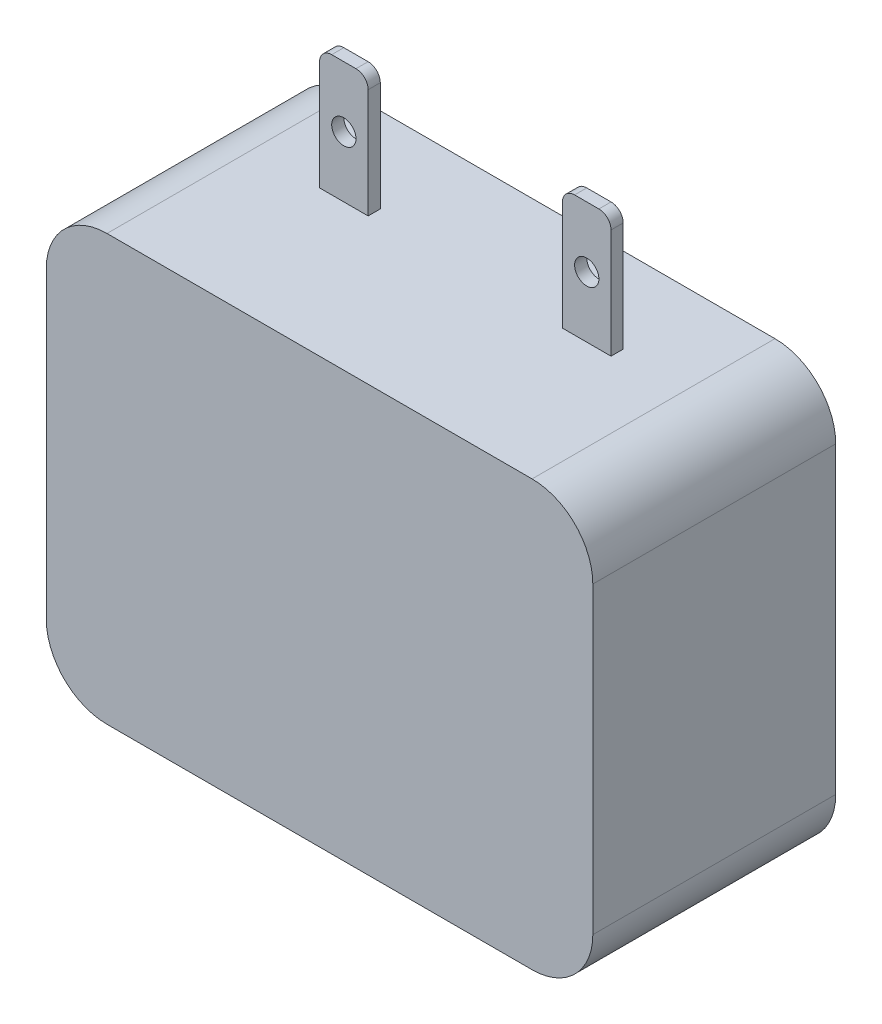
SolidWorks part; units mm, degrees
ref_plane "Front Plane" through (0, 0, 0) normal (0, 0, 1) x (1, 0, 0)
ref_plane "Top Plane" through (0, 0, 0) normal (0, 1, 0) x (1, 0, 0)
ref_plane "Right Plane" through (0, 0, 0) normal (1, 0, 0) x (0, 0, -1)
sketch "Sketch1" plane through (0, 0, 0) normal (0, 0, 1) x (1, 0, 0)
  line L1 (-17.5, -17.5) -> (17.5, -17.5)
  line L2 (-22.5, -12.5) -> (-22.5, 12.5)
  line L3 (-17.5, 17.5) -> (17.5, 17.5)
  line L4 (22.5, -12.5) -> (22.5, 12.5)
  line L5 (-22.5, -17.5) -> (22.5, 17.5) construction
  line L6 (-22.5, 17.5) -> (22.5, -17.5) construction
  arc A0 (-17.5, -17.5) -> (-22.5, -12.5) centre (-17.5, -12.5) cw
  arc A1 (17.5, -17.5) -> (22.5, -12.5) centre (17.5, -12.5) ccw
  arc A2 (17.5, 17.5) -> (22.5, 12.5) centre (17.5, 12.5) cw
  arc A3 (-22.5, 12.5) -> (-17.5, 17.5) centre (-17.5, 12.5) cw
  point P0 (0, 0)
  dimension "D3" = 5
  dimension "D1" = 35
  dimension "D2" = 45
extrude "Boss-Extrude1" add sketch "Sketch1" along normal mid plane 20
ref_plane "Plane1" through (0, 0, -3) normal (0, 0, -1) x (-1, 0, 0)
sketch "Sketch3" plane through (0, 0, -3) normal (0, 0, -1) x (-1, 0, 0)
  line L0 (-17.5, 17.5) -> (17.5, 17.5) construction
  line L4 (-8, 17.5) -> (-12, 17.5)
  line L5 (-8, 17.5) -> (-8, 26.5)
  line L6 (-9, 27.5) -> (-11, 27.5)
  line L7 (-12, 17.5) -> (-12, 26.5)
  line L8 (0, 11) -> (0, -11) construction
  line L9 (8, 17.5) -> (12, 17.5)
  line L10 (9, 27.5) -> (11, 27.5)
  line L11 (8, 17.5) -> (8, 26.5)
  line L12 (12, 17.5) -> (12, 26.5)
  line L13 (17.5, -17.5) -> (-17.5, -17.5) construction
  line L14 (-2.5, -17.5) -> (2.5, -17.5)
  line L15 (-2.5, -17.5) -> (-2.5, -26.5)
  line L16 (-1.5, -27.5) -> (1.5, -27.5)
  line L17 (2.5, -17.5) -> (2.5, -26.5)
  arc A2 (-8, 26.5) -> (-9, 27.5) centre (-9, 26.5) ccw
  arc A3 (-11, 27.5) -> (-12, 26.5) centre (-11, 26.5) ccw
  arc A4 (11, 27.5) -> (12, 26.5) centre (11, 26.5) cw
  arc A5 (8, 26.5) -> (9, 27.5) centre (9, 26.5) cw
  arc A6 (-2.5, -26.5) -> (-1.5, -27.5) centre (-1.5, -26.5) ccw
  arc A7 (1.5, -27.5) -> (2.5, -26.5) centre (1.5, -26.5) ccw
  circle A8 centre (0, -22.5) radius 1
  point P8 (-8, 27.5)
  point P11 (-12, 27.5)
  point P29 (0, -27.5)
  point P32 (-2.5, -27.5)
  point P35 (2.5, -27.5)
  dimension "D1" = 10
  dimension "D4" = 1
  dimension "D7" = 1
  dimension "D9" = 2
  dimension "D2" = 4
  dimension "D3" = 8
  dimension "D5" = 5
  dimension "D6" = 10
  dimension "D8" = 5
extrude "Boss-Extrude2" add sketch "Sketch3" against normal blind 1
sketch "Sketch4" plane through (0, 0, -3) normal (0, 0, -1) x (-1, 0, 0)
  line L0 (11, 27.5) -> (9, 27.5) construction
  line L1 (-9, 27.5) -> (-11, 27.5) construction
  line L2 (-17.5, 17.5) -> (17.5, 17.5) construction
  circle A0 centre (-10, 22.5) radius 1
  circle A1 centre (10, 22.5) radius 1
  point P7 (10, 27.5)
  point P10 (-10, 27.5)
  dimension "D1" = 2
  dimension "D2" = 2
  dimension "D3" = 5
extrude "Cut-Extrude1" cut sketch "Sketch4" against normal blind 1
